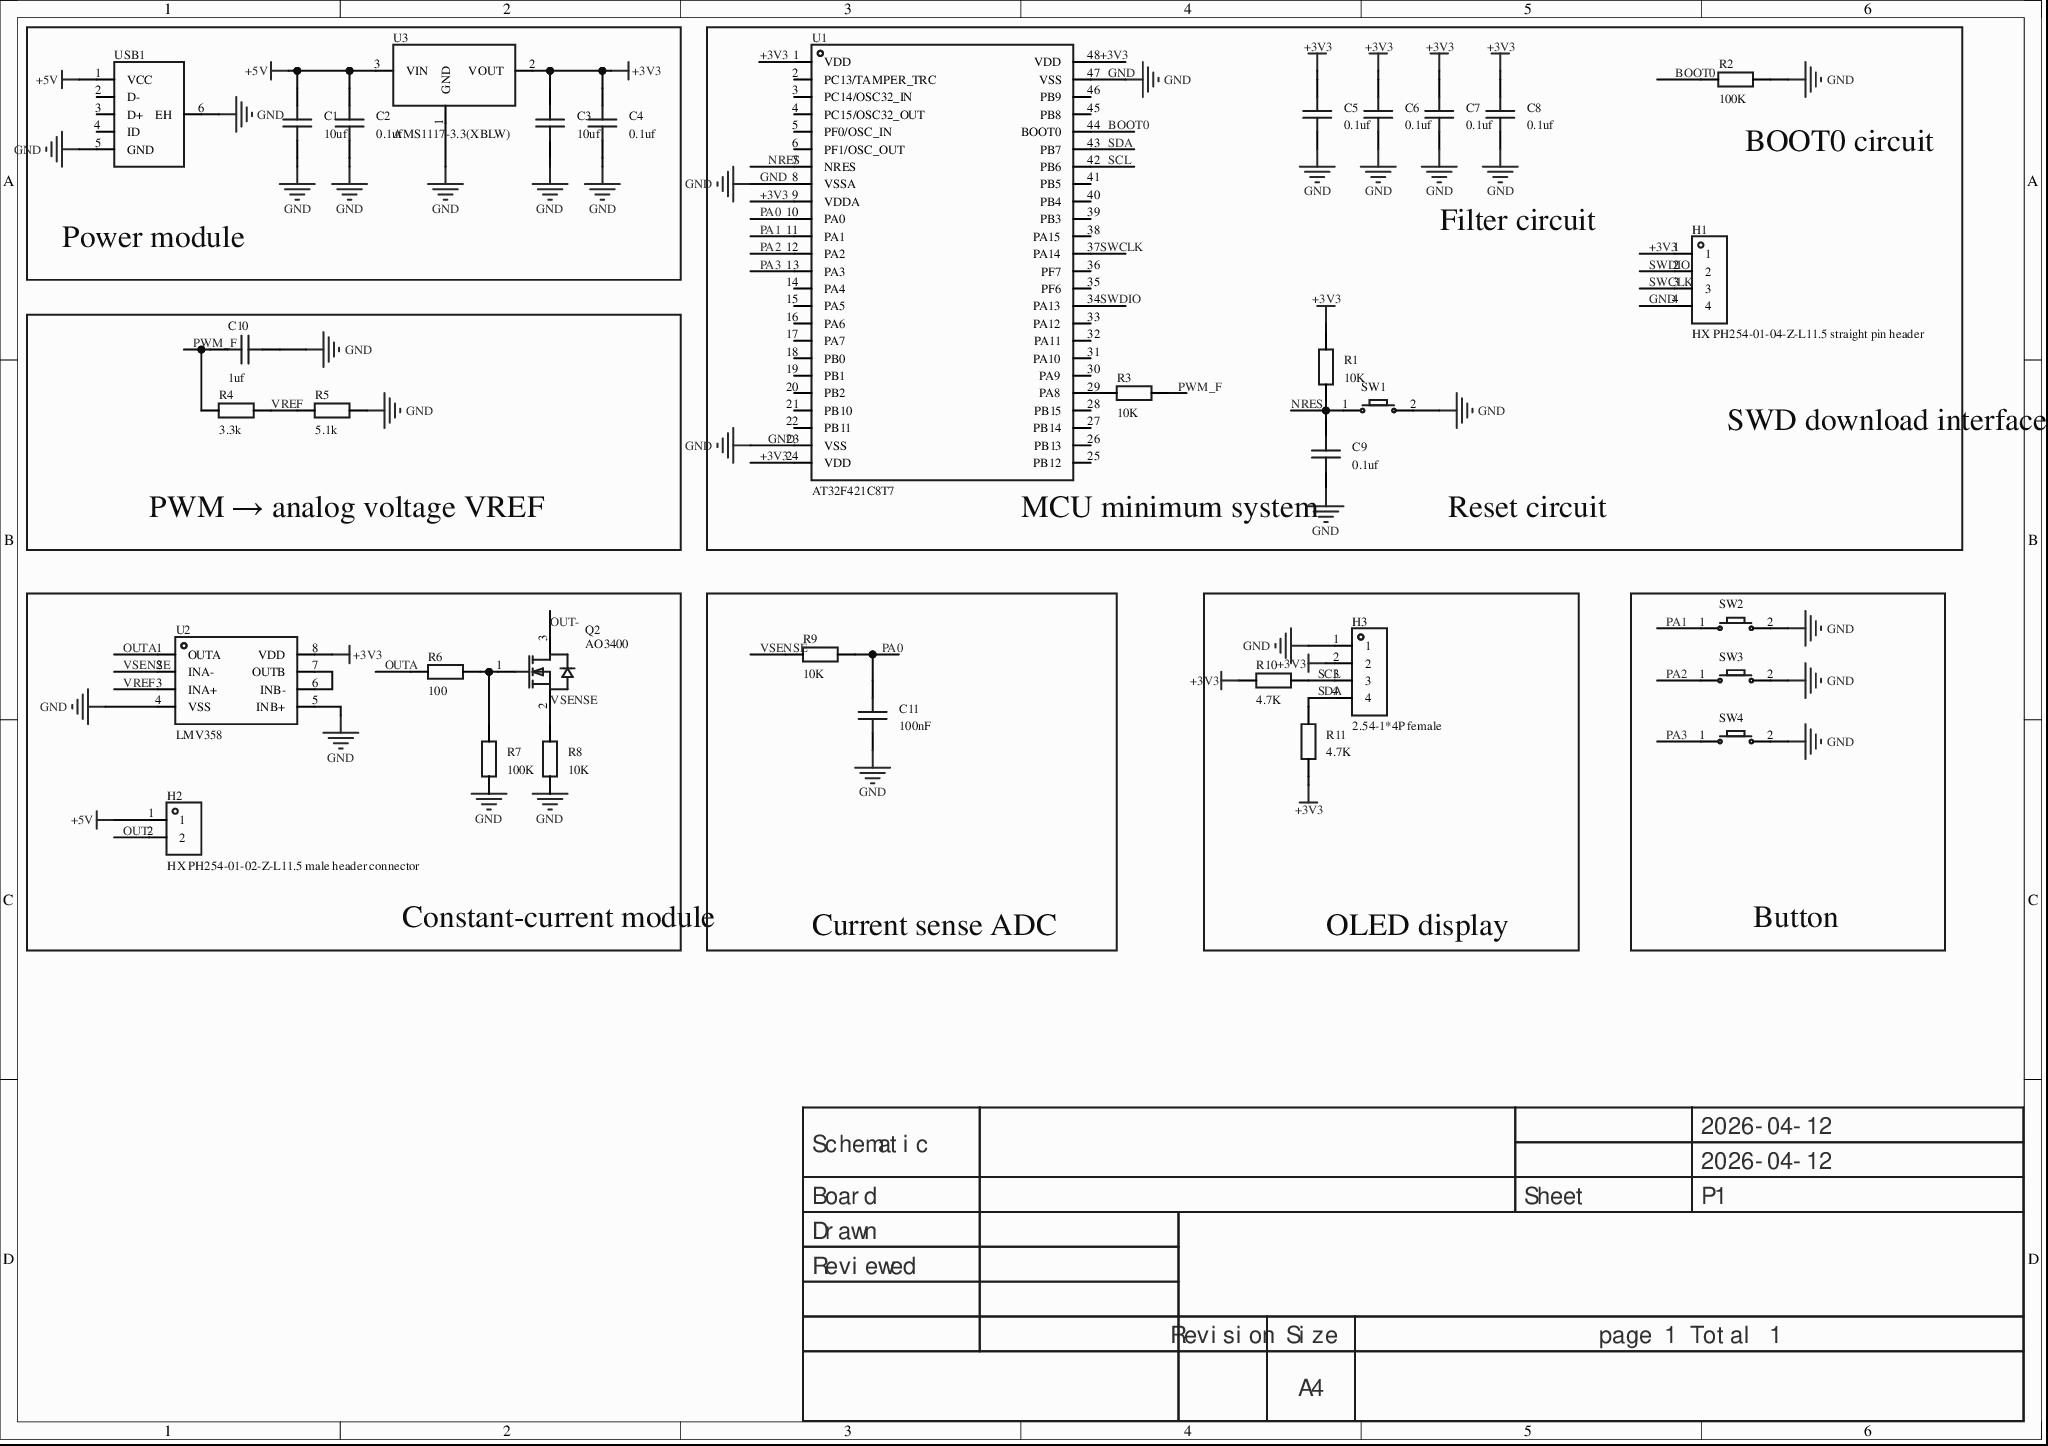
[diagram p0: MISC52008-3.schdoc]
# Altium project MISC52008-2.PrjPcb
1 sheet, 34 parts. Net scope: global (net labels, ports and power ports of the same name join across sheets).
Board file: MISC52008.pcbdoc

## Sheet MISC52008-3.schdoc
size 297 x 209 mm; Version: V1.0; @Project Name: MISC52008; @Update Date: 2026-04-12; @Create Date: 2026-04-12; @Board Name: MISC52008; @Create Time: 17:23:53; @Page Count: 1; @Page No: 1; @Schematic Name: MISC52008; @Update Time: 17:23:53; Size: A4

### Parts
C1  10uf  [C0603]
C2  0.1uf  [C0603]
C3  10uf  [C0603]
C4  0.1uf  [C0603]
C5  0.1uf  [C0603]
C6  0.1uf  [C0603]
C7  0.1uf  [C0603]
C8  0.1uf  [C0603]
C9  0.1uf  [C0603]
C10  1uf  [C0603]
C11  100nF  [C0603]
H1  HX PH254-01-04-Z-L11.5 straight pin header  [HDR-TH_4P-HX-PH254-01-04-Z-L11.5]
H2  HX PH254-01-02-Z-L11.5 male header connector  [HDR-TH_2P-P2.54-V-M]
H3  2.54-1*4P female  [HDR-TH_4P-P2.54-V-F]
Q2  AO3400  [SOT-23_L2.9-W1.3-P1.90-LS2.4-BR]
R1  10K  [R0603]
R2  100K  [R0603]
R3  10K  [R0603]
R4  3.3k  [R0603]
R5  5.1k  [R0603]
R6  100  [R0603]
R7  100K  [R0603]
R8  10K  [R0603]
R9  10K  [R0603]
R10  4.7K  [R0603]
R11  4.7K  [R0603]
SW1  (no value)  [Key_SMD_3x4x2]
SW2  (no value)  [Key_SMD_3x4x2]
SW3  (no value)  [Key_SMD_3x4x2]
SW4  (no value)  [Key_SMD_3x4x2]
U1  AT32F421C8T7  [LQFP-48_L7.0-W7.0-P0.50-LS9.0-BL]
U2  LMV358  [SOP-8_L4.9-W3.9-P1.27-LS6.0-BL]
U3  AMS1117-3.3(XBLW)  [SOT-223-3_L6.5-W3.4-P2.30-LS7.0-BR-1]
USB1  (no value)  [USB_Micro]

### Blocks framed on the sheet
Power module: C1-C4 U3 USB1
PWM → analog voltage VREF: C10 R4 R5
Constant-current module: H2 Q2 R6-R8 U2
Current sense ADC: C11 R9
OLED display: H3 R10 R11
Button: SW2-SW4

### Nets
+3V3: C3.2 C4.2 C5.2 C6.2 C7.2 C8.2 H1.1 H3.2 R1.2 R10.1 R11.1 U1.1(VDD) U1.9(VDDA) U1.24(VDD) U1.48(VDD) U2.8(VDD) U3.2(VOUT)
+5V: C1.2 C2.2 H2.1 U3.3(VIN) USB1.1(VCC)
GND: C1.1 C2.1 C3.1 C4.1 C5.1 C6.1 C7.1 C8.1 C9.1 C10.2 C11.1 H1.4 H3.1 R2.2 R5.2 R7.1 R8.1 SW1.2 SW2.2 SW3.2 SW4.2 U1.8(VSSA) U1.23(VSS) U1.47(VSS) U2.4(VSS) U2.5(INB+) U3.1(GND) USB1.5(GND) USB1.6(EH)
BOOT0: R2.1 U1.44(BOOT0)
NRES: C9.2 R1.1 SW1.1 U1.7(NRES)
OUT-: H2.2 Q2.3(D)
OUTA: R6.1 U2.1(OUTA)
PA0: C11.2 R9.2 U1.10(PA0)
PA1: SW2.1 U1.11(PA1)
PA2: SW3.1 U1.12(PA2)
PA3: SW4.1 U1.13(PA3)
PWM_F: C10.1 R3.2 R4.1
SCL: H3.3 R10.2 U1.42(PB6)
SDA: H3.4 R11.2 U1.43(PB7)
SWCLK: H1.3 U1.37(PA14)
SWDIO: H1.2 U1.34(PA13)
VREF: R4.2 R5.1 U2.3(INA+)
VSENSE: Q2.2(S) R8.2 R9.1 U2.2(INA-)
NetQ2_1: Q2.1(G) R6.2 R7.2
NetR3_1: R3.1 U1.29(PA8)
NetU2_6: U2.6(INB-) U2.7(OUTB)

Not connected (* = marked no-connect by the designer): U1 2(PC13/TAMPER_TRC)* 3(PC14/OSC32_IN)* 4(PC15/OSC32_OUT)* 5(PF0/OSC_IN)* 6(PF1/OSC_OUT)* 14(PA4)* 15(PA5)* 16(PA6)* 17(PA7)* 18(PB0)* 19(PB1)* 20(PB2)* 21(PB10)* 22(PB11)* 25(PB12)* 26(PB13)* 27(PB14)* 28(PB15)* 30(PA9)* 31(PA10)* 32(PA11)* 33(PA12)* 35(PF6)* 36(PF7)* 38(PA15)* 39(PB3)* 40(PB4)* 41(PB5)* 45(PB8)* 46(PB9)*; USB1 2(D-)* 3(D+)* 4(ID)*

### Notes on the sheet
- (near R2) BOOT0 circuit
- (near H1) Filter circuit
- SWD download interface
- MCU minimum system
- Reset circuit
- 2026-04-12
- Schematic
- Board
- Sheet
- P1
- Drawn
- Reviewed
- Revision
- Size
- A4
- page 1 Total 1

### Library data of the parts
C1-C9 = CAP_0603: Symbol: Capacitance; ConvertToPcb: yes; ModelId: ac125912035d415993ca9572d50418b10819f05c4eef4c71ace90d822a990e87; ModelName: C0603_L1.6-W0.8-H0.8; ModelTransform: 62.992,31.496,0,0,0,0,0,0,0; Device: CAP_0603; AddInBom: yes; Supplier Footprint: 0603; FootprintName: C0603
  C1 C3: Value: 10uf
  C2 C4-C9: Value: 0.1uf
C10 C11 = CAP_0603: Symbol: Capacitance; 3D Model: ac125912035d415993ca9572d50418b10819f05c4eef4c71ace90d822a990e87; 3D Model Transform: 62.992,31.496,0,0,0,0,0,0,0; ConvertToPcb: yes; ModelName: C0603_L1.6-W0.8-H0.8; Device: CAP_0603; Supplier Footprint: 0603; AddInBom: yes; FootprintName: C0603
  C10: Value: 1uf
  C11: Value: 100nF
H1 = HX PH254-01-04-Z-L11.5 straight pin header: 插针结构:1x4P;间距:2.54mm;圆针/方针:方针;安装方式:直插;排数:单排;总PIN位数:4P;额定电流:3A;额定电压:1kV;配合针长度:6mm;塑高:2.5mm;端接针长度:3mm;触头材质:黄铜;触头镀层:金;工作温度:-40℃~+105℃;; Manufacturer: hanxia(韩下); AddInBom: yes; ModelId: 8a04245d30e54eb999146b73785c6ab00819f05c4eef4c71ace90d822a990e87; ModelTransform: 392.519,98.425,0,0,0,0,0,0,-118.11; Pin Structure: 1x4P; Pitch: 2.54mm; Circluar Pins/Square Pins: Square pin; Current Rating: 3A; Voltage Rating (Max): 1kV; Symbol: HX PH254-01-04-Z-L11.5 STRAIGHT PIN HEADER; Device: HX PH254-01-04-Z-L11.5 straight pin header; LCSC Part Name: 1x4P 间距:2.54mm 方针 直插; SupplierPart: C52016392; ManufacturerPart: HX PH254-01-04-Z-L11.5 straight pin header; Supplier Footprint: 插件,P=2.54mm; JLCPCB Part Class: Extended Part; Datasheet: https://item.szlcsc.com/datasheet/HX%2520PH254-01-04-Z-L11.5%2520straight%2520pin%2520header/54760437.html; Supplier: LCSC; ConvertToPcb: yes; FootprintName: HDR-TH_4P-HX-PH254-01-04-Z-L11.5; ModelName: HDR-TH_4P-HX-PH254-01-04-Z-L11.5; Mounting Type: Through-hole; Number of Rows: Single row; Number of Pins: 4P; Length of Mating Pin: 6mm; Insulation Height: 2.5mm; Length of End Connection Pin: 3mm; Contact Material: Brass; Contact Plating: Gold; Operating Temperature: -40℃~+105℃
H2 = HX PH254-01-02-Z-L11.5 male header connector: 插针结构:1x2P;间距:2.54mm;圆针/方针:方针;安装方式:直插;排数:单排;总PIN位数:2P;额定电流:3A;额定电压:1kV;配合针长度:6mm;塑高:2.5mm;端接针长度:3mm;触头材质:黄铜;触头镀层:金;工作温度:-40℃~+105℃;; Manufacturer: hanxia(韩下); AddInBom: yes; ModelId: e35305ec3aa84b66b849f914b715e73f0819f05c4eef4c71ace90d822a990e87; ModelName: HDR2.54-M-LI-1X2P; ModelTransform: 200,100,0,0,0,0,0,0,-118.11; Pin Structure: 1x2P; Pitch: 2.54mm; Circluar Pins/Square Pins: Square pin; Current Rating: 3A; Voltage Rating (Max): 1kV; Symbol: HX PH254-01-02-Z-L11.5 MALE HEADER CONNECTOR; Device: HX PH254-01-02-Z-L11.5 male header connector; LCSC Part Name: 1x2P 间距:2.54mm 方针 直插; SupplierPart: C52016390; ManufacturerPart: HX PH254-01-02-Z-L11.5 male header connector; Supplier Footprint: 插件,P=2.54mm; JLCPCB Part Class: Extended Part; Datasheet: https://item.szlcsc.com/datasheet/HX%2520PH254-01-02-Z-L11.5%2520male%2520header%2520connector/54760435.html; Supplier: LCSC; ConvertToPcb: yes; FootprintName: HDR-TH_2P-P2.54-V-M; Mounting Type: Through-hole; Number of Rows: Single row; Number of Pins: 2P; Length of Mating Pin: 6mm; Insulation Height: 2.5mm; Length of End Connection Pin: 3mm; Contact Material: Brass; Contact Plating: Gold; Operating Temperature: -40℃~+105℃
H3 = 2.54-1*4P母: 插孔结构:1x4P;间距:2.54mm;行距:-;圆孔/方孔:方孔;安装方式:直插;排数:单排;总孔位数:4P;额定电流:3A;额定电压:-;插孔方向:顶部;塑高:-;触头材质:青铜;触头镀层:-;工作温度:-40℃~+105℃;; Manufacturer: BOOMELE(博穆精密); AddInBom: yes; ModelId: d187812051054f85879fcaa51a310d8e0819f05c4eef4c71ace90d822a990e87; ModelTransform: 419.6842,98.464,0,0,0,0,0,0,-118.11; Holes Structure: 1x4P; Pitch: 2.54mm; Circular Hole / Square Hole: Square hole; Number of Positions: 4P; Current Rating: 3A; Holes Direction: Top; Symbol: 2.54-1*4P female; Device: 2.54-1*4P female; LCSC Part Name: 间距:2.54mm 1x4P 直插; SupplierPart: C2718488; ManufacturerPart: 2.54-1*4P母; Supplier Footprint: 插件,P=2.54mm; JLCPCB Part Class: Extended Part; Datasheet: https://item.szlcsc.com/datasheet/2.54-1*4P%25E6%25AF%258D/2834502.html; Supplier: LCSC; ConvertToPcb: yes; FootprintName: HDR-TH_4P-P2.54-V-F; ModelName: HDR-TH_4P-P2.54-V-F; Row Spacing: -; Mounting Type: Through-hole; Number of Rows: Single row; Voltage Rating (Max): -; Insulation Height: -; Contact Material: Bronze; Contact Plating: -; Operating Temperature: -40℃~+105℃
Q2 = AO3400_C2938367: 数量:1个N沟道;漏源电压(Vdss):30V;连续漏极电流(Id):5.8A;导通电阻(RDS(on)):28mΩ@10V;耗散功率(Pd):1.5W;阈值电压(Vgs(th)):1.4V@250uA;; Manufacturer: GOODWORK(固得沃克); AddInBom: yes; ModelId: c62791f0466c4ae2a892c056b845b0ca0819f05c4eef4c71ace90d822a990e87; ModelName: SOT-23-3P_L2.9-W1.3-H1.0-LS2.4-P0.95; ModelTransform: 98.64468,114.173,0,180,0,0,0.001,-0.002,0; Number: 1 N-channel; Drain to Source Voltage: 30V; Current - Continuous Drain(Id): 5.8A; Pd - Power Dissipation: 1.5W; Input Capacitance(Ciss): 1.05nF; Reverse Transfer Capacitance (Crss@Vds): 77pF@15V; Type: N-channel; Symbol: AO3400_C2938367; Device: AO3400_C2938367; LCSC Part Name: 1个N沟道 耐压:30V 电流:5.8A; SupplierPart: C2938367; ManufacturerPart: AO3400; Supplier Footprint: SOT-23; JLCPCB Part Class: Extended Part; Datasheet: https://item.szlcsc.com/datasheet/AO3400/3294704.html; Supplier: LCSC; ConvertToPcb: yes; FootprintName: SOT-23_L2.9-W1.3-P1.90-LS2.4-BR; RDS(on): 28mΩ@10V; Gate Threshold Voltage (Vgs(th)): 1.4V@250uA; Gate Charge(Qg): -; Operating Temperature: -55℃~+150℃
R1 R2 = Res_0603: Symbol: Resistor; ConvertToPcb: yes; ModelId: fc143cca1e79419f9cd78b61e9279f080819f05c4eef4c71ace90d822a990e87; ModelTransform: 31.8897,63.7794,0,90,0,0,0,0,0; Device: Res_0603; AddInBom: yes; Supplier Footprint: 0603; FootprintName: R0603; ModelName: R0603
  R1: Value: 10K
  R2: Value: 100K
R3-R11 = Res_0603: Symbol: Resistor; 3D Model: fc143cca1e79419f9cd78b61e9279f080819f05c4eef4c71ace90d822a990e87; 3D Model Transform: 31.8897,63.7794,0,90,0,0,0,0,0; ConvertToPcb: yes; Device: Res_0603; Supplier Footprint: 0603; AddInBom: yes; FootprintName: R0603; ModelName: R0603
  R3 R8 R9: Value: 10K
  R4: Value: 3.3k
  R5: Value: 5.1k
  R6: Value: 100
  R7: Value: 100K
  R10 R11: Value: 4.7K
SW1-SW4 = Key_SMD_3x4x2: Symbol: Tactile switch x2; ConvertToPcb: yes; ModelId: 63599cce708d48afbce1b0db003544770819f05c4eef4c71ace90d822a990e87; ModelName: SW-SMD_L4.0-W2.9-H2-LS5.0; ModelTransform: 196.85,114.17,79.13,0,0,0,0,0,0; Device: Key_SMD_3x4x2; AddInBom: yes; Supplier Footprint: SMD; FootprintName: Key_SMD_3x4x2
U1 = AT32F421C8T7: CPU内核:CM4;程序存储容量:64KB;RAM总容量:16KB;GPIO端口数量:-;工作电压范围:-;CPU最大主频:-;程序存储器类型:FLASH;; Manufacturer: ARTERY(雅特力); AddInBom: yes; ModelId: 093be70396ff421eb2cdb946d5311efc0819f05c4eef4c71ace90d822a990e87; ModelName: LQFP-48_L7.0-W7.0-H1.4-LS9.0-P0.50; ModelTransform: 354.331,354.331,0,0,0,0,0,0,0; CPU Core: CM4; Program Storage Size: 64KB; RAM Size: 16KB; Program Memory Type: FLASH; Symbol: AT32F421C8T7; Device: AT32F421C8T7; LCSC Part Name: AT32F421C8T7; SupplierPart: C2687447; ManufacturerPart: AT32F421C8T7; Supplier Footprint: LQFP-48(7x7); JLCPCB Part Class: Extended Part; Datasheet: https://atta.szlcsc.com/upload/public/pdf/source/20210622/C2765098_2C72C7B1BCEA7473D7B0BCEAEE10BC9B.pdf; Supplier: LCSC; ConvertToPcb: yes; FootprintName: LQFP-48_L7.0-W7.0-P0.50-LS9.0-BL; GPIO Ports Number: -; Operating Voltage Range: -; CPU Maximum Speed: -; ADC (Bit): -; DAC (Bit): -; PWM (Bit): -; Universal Serial Bus: -; Internal Comparator: -; communication protocol: -; Watchdog: -; Real-Time Clock: -; Infrared Data Association: -; Low-Voltage Detect: -; CCP Capture/Compare: -; Secure Digital Input and Output: -; Direct Memory Access: -; Internal Oscillator: Yes
U2 = LMV358: 放大器数:2;轨到轨:轨到轨输入,轨到轨输出;增益带宽积(GBW):1MHz;输入失调电压(Vos):5mV;压摆率(SR):600V/ms;输入偏置电流(Ib):10pA;; Manufacturer: TECH PUBLIC(台舟); Symbol: LMV358_C2923376; AddInBom: yes; ModelId: 75c24a7891ee4dd6bdac16a7163ff87e0819f05c4eef4c71ace90d822a990e87; ModelName: SOP-8_L4.9-W3.9-P1.27-LS6.0-BL-1; ModelTransform: 192.913,236.22,0,0,0,0,0,0,0; Number of Channels: 2; Maximum Power Supply Range (Vdd-Vss): 5.5V; Rail to Rail: Rail-to-rail input, rail-to-rail output; Gain Bandwidth Product: 1MHz; Vos - Input Offset Voltage: 5mV; Input Offset Voltage Drift(Vos TC): 2uV/℃; Ib - Input Bias Current: 10pA; Input Voltage Noise Density: 20nV/√Hz@10kHz; Common Mode Rejection Ratio(CMRR): 65dB; Quiescent Current: 40uA; Output Current: 20mA; Single supply: 2.5V~5.5V; Device: LMV358; LCSC Part Name: CMOS，轨到轨通用放大器; SupplierPart: C2923376; ManufacturerPart: LMV358; Supplier Footprint: SOP-8; JLCPCB Part Class: Extended Part; Datasheet: https://item.szlcsc.com/datasheet/LMV358/3234834.html; Supplier: LCSC; ConvertToPcb: yes; FootprintName: SOP-8_L4.9-W3.9-P1.27-LS6.0-BL; Slew Rate: 600V/ms; Input Offset Current(Ios): 10pA; Input offset current drift(Ios TC): -; Operating Temperature: -40℃~+125℃; Dual Supply: -; Features: -
U3 = AMS1117-3.3(XBLW): Output type: fixed; max input voltage: 15V; output voltage: 3.3V; output current: 1A; power supply rejection ratio (PSRR): 60dB; output polarity: positive;; Manufacturer: XBLW(芯伯乐); Symbol: AMS1117-3.3(XBLW)_C18906017; AddInBom: yes; ModelId: 0a360ebfdb9248a182f670f5fd8a68d20819f05c4eef4c71ace90d822a990e87; ModelTransform: 275.59,255.905,0,0,0,0,-3.937,0,0; Dropout Voltage: 1.3V; standby current: 4mA; Number of Outputs: 1; Device: AMS1117-3.3(XBLW); LCSC Part Name: AMS1117-3.3(XBLW); SupplierPart: C18906017; ManufacturerPart: AMS1117-3.3(XBLW); Supplier Footprint: SOT-223; JLCPCB Part Class: Extended Part; Datasheet: https://atta.szlcsc.com/upload/public/pdf/source/20231019/F4230EEFC48908FC91962BB59ACA9AD6.pdf; Supplier: LCSC; ConvertToPcb: yes; FootprintName: SOT-223-3_L6.5-W3.4-P2.30-LS7.0-BR-1; ModelName: SOT-223-3_L6.5-W3.4-P2.30-LS7.0-BR-1; Output Type: Fixed; Maximum Input Voltage: 15V; Output Voltage: 3.3V; Output Current: 1A; Power Supply Rejection Ratio (PSRR): 60dB; Noise: -; Feature: Thermal protection (TSD); overcurrent protection (OCP); Operating Temperature: -40℃~+125℃; Output Polarity: Positive
USB1 = USB_Micro-B: AddInBom: yes; ModelId: 4933c3c2baea4358bc2662474c6970960819f05c4eef4c71ace90d822a990e87; ModelName: MINI-USB-SMD_MICRO-4P-DIP; ModelTransform: 295.275,240.157,0,180,0,0,0,-34.253,-39.37; Symbol: USB_Micro; Device: USB_Micro-B; ConvertToPcb: yes; FootprintName: USB_Micro; Supplier Footprint: SMD